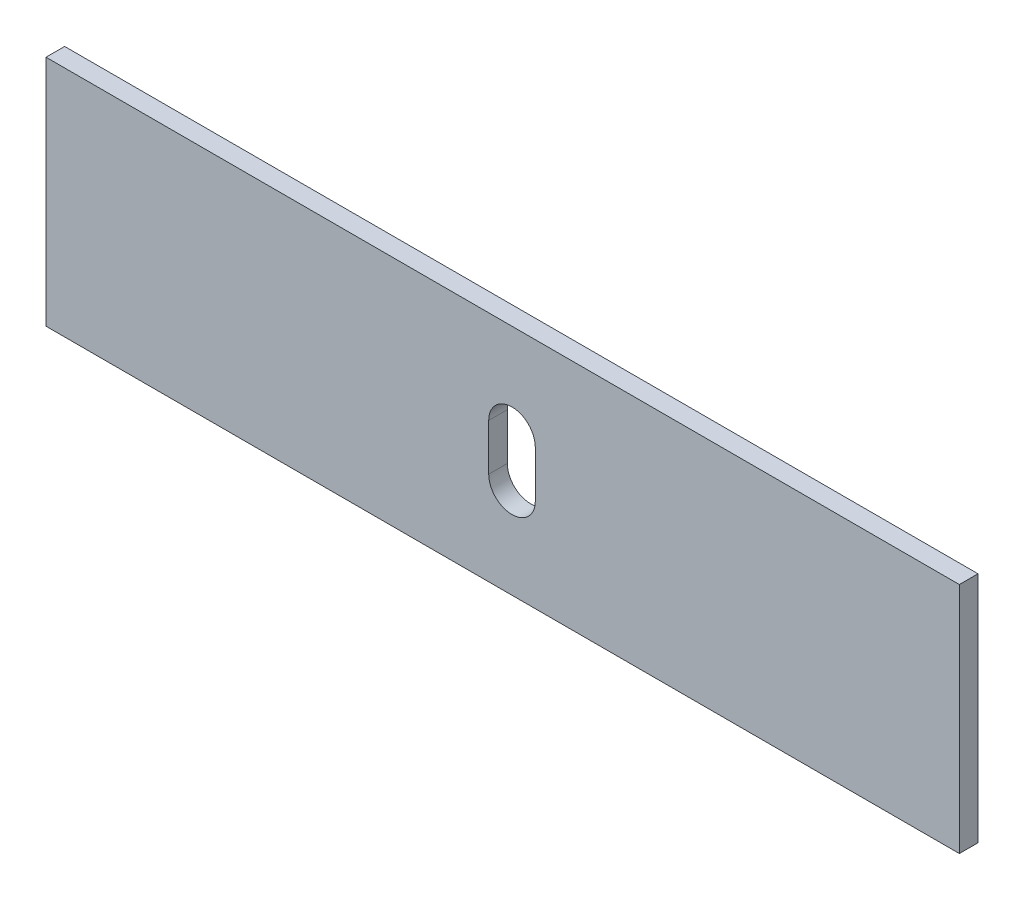
from build123d import *

# Parameters (mm, degrees)
BOSS_EXTRUDE1_DEPTH = 20


with BuildPart() as part:
    # Sketch1 → Boss-Extrude1 (new body)
    with BuildSketch(Plane.XY):
        Polygon((11341.12511676, 4637.824188368), (11341.125116846, 4387.824188368), (12321.125115149, 4387.824188368), (12321.125115149, 4637.824188368), align=None)
        with BuildLine():
            Line((11816.125116094, 4537.824187896), (11816.125116094, 4487.824187992))
            ThreePointArc((11816.125116094, 4487.824187992), (11841.125216971, 4462.824188038), (11866.125116001, 4487.824389839))
            Line((11866.125116001, 4487.824389839), (11866.125116001, 4537.823600328))
            ThreePointArc((11866.125116001, 4537.823600328), (11841.125409832, 4562.823894066), (11816.125116094, 4537.824187896))
        make_face(mode=Mode.SUBTRACT)
    extrude(amount=BOSS_EXTRUDE1_DEPTH)


solid = part.part
